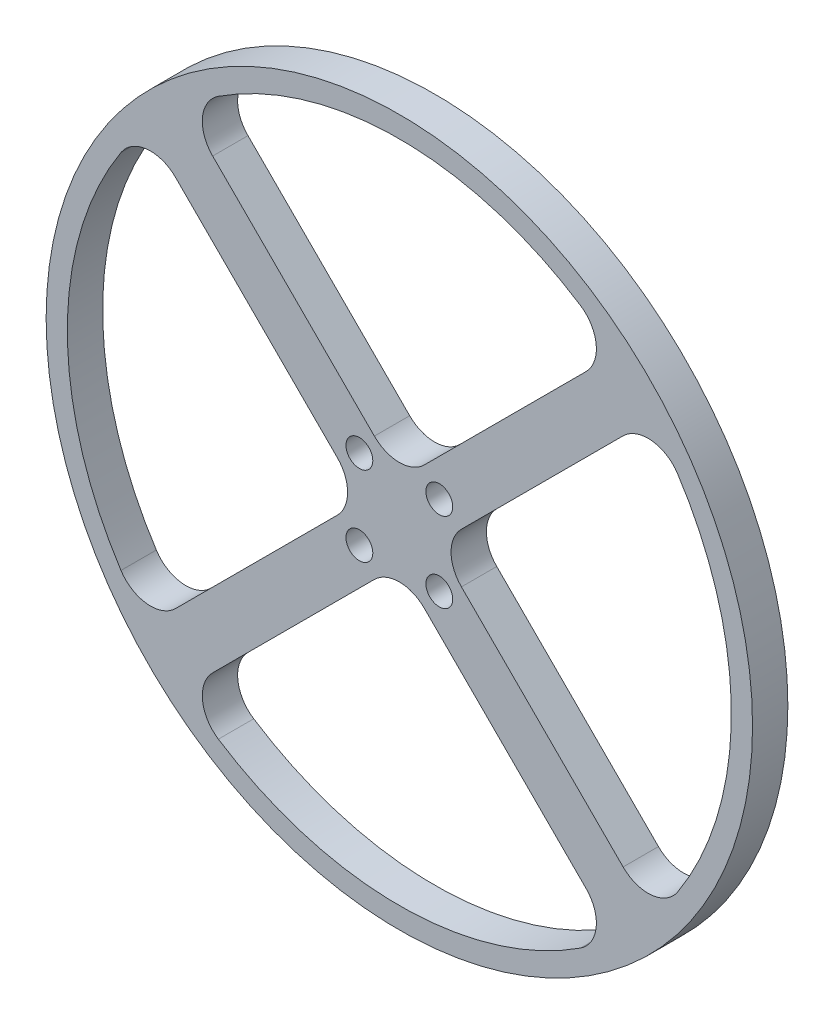
from build123d import *

# Parameters (mm, degrees)
SKETCH1_R           = 50
BOSS_EXTRUDE1_DEPTH = 5
FILLET1_R           = 5
SKETCH2_R           = 1.9
CUT_EXTRUDE1_DEPTH  = 5


with BuildPart() as part:
    # Sketch1 → Boss-Extrude1 (new body)
    with BuildSketch(Plane.XY):
        Circle(SKETCH1_R)
        with BuildLine():
            Line((30.504506916, 35.755769574), (0, 5.251262658))
            Line((0, 5.251262658), (-30.504506916, 35.755769574))
            ThreePointArc((-30.504506916, 35.755769574), (0, 47), (30.504506916, 35.755769574))
        make_face(mode=Mode.SUBTRACT)
        with BuildLine():
            Line((5.251262658, 0), (35.755769574, 30.504506916))
            ThreePointArc((35.755769574, 30.504506916), (47, 0), (35.755769574, -30.504506916))
            Line((35.755769574, -30.504506916), (5.251262658, 0))
        make_face(mode=Mode.SUBTRACT)
        with BuildLine():
            Line((0, -5.251262658), (30.504506916, -35.755769574))
            ThreePointArc((30.504506916, -35.755769574), (0, -47), (-30.504506916, -35.755769574))
            Line((-30.504506916, -35.755769574), (0, -5.251262658))
        make_face(mode=Mode.SUBTRACT)
        with BuildLine():
            Line((-5.251262658, 0), (-35.755769574, -30.504506916))
            ThreePointArc((-35.755769574, -30.504506916), (-47, 0), (-35.755769574, 30.504506916))
            Line((-35.755769574, 30.504506916), (-5.251262658, 0))
        make_face(mode=Mode.SUBTRACT)
    extrude(amount=BOSS_EXTRUDE1_DEPTH)

    # Fillet1
    fillet1_edges = [part.edges().sort_by_distance(p)[0] for p in [
        (-5.251262658, 0, 2.5),
        (-35.755769574, 30.504506916, 2.5),
        (-35.755769574, -30.504506916, 2.5),
        (35.755769574, -30.504506916, 2.5),
        (35.755769574, 30.504506916, 2.5),
        (5.251262658, 0, 2.5),
        (-30.504506916, -35.755769574, 2.5),
        (30.504506916, -35.755769574, 2.5),
        (0, -5.251262658, 2.5),
        (30.504506916, 35.755769574, 2.5),
        (-30.504506916, 35.755769574, 2.5),
        (0, 5.251262658, 2.5),
    ]]
    fillet(fillet1_edges, radius=FILLET1_R)

    # Sketch2 → Cut-Extrude1 (cut)
    with BuildSketch(Plane.XY.offset(5)):
        with Locations((5.656854249, -5.656854249)):
            Circle(SKETCH2_R)
        with Locations((5.656854249, 5.656854249)):
            Circle(SKETCH2_R)
        with Locations((-5.656854249, 5.656854249)):
            Circle(SKETCH2_R)
        with Locations((-5.656854249, -5.656854249)):
            Circle(SKETCH2_R)
    extrude(amount=-CUT_EXTRUDE1_DEPTH, mode=Mode.SUBTRACT)


solid = part.part
